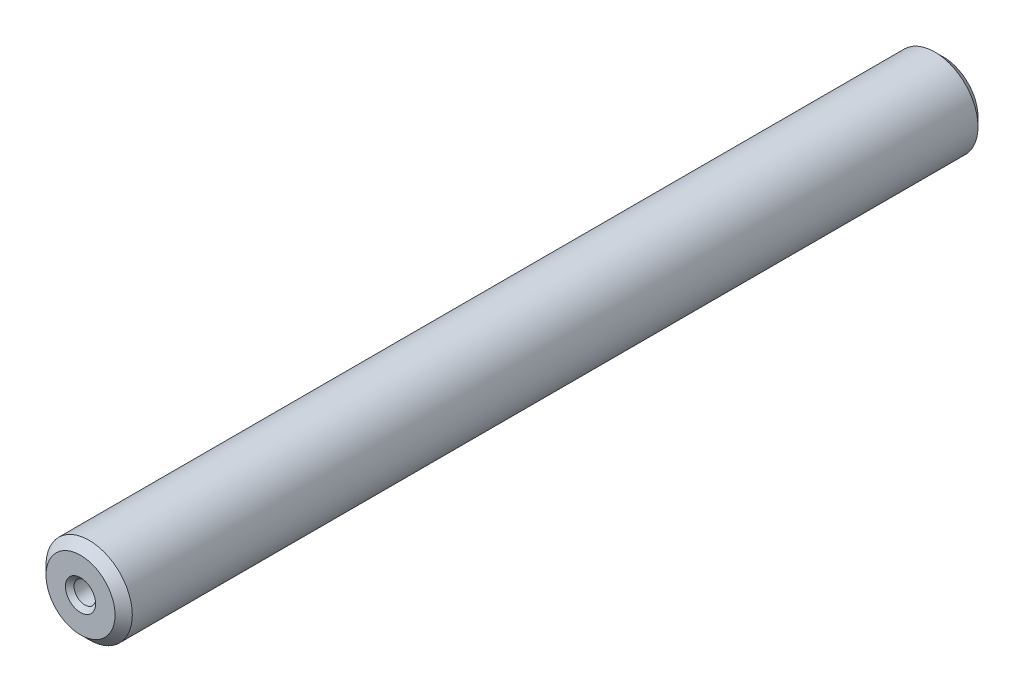
from build123d import *

# Parameters (mm, degrees)
SKETCH1_R             = 5
BOSS_EXTRUDE1_DEPTH   = 100
M3_TAPPED_HOLE1_D     = 2.5
M3_TAPPED_HOLE1_DEPTH = 6.5
M3_TAPPED_HOLE1_TIP   = 0.751075774
CHAMFER1_SIZE         = 1
CHAMFER2_SIZE         = 0.5


with BuildPart() as part:
    # Sketch1 → Boss-Extrude1 (new body)
    with BuildSketch(Plane.XY):
        Circle(SKETCH1_R)
    extrude(amount=BOSS_EXTRUDE1_DEPTH)

    # M3 Tapped Hole1
    with Locations(Plane.XY.offset(100)):
        with Locations((0, 0)):
            Hole(M3_TAPPED_HOLE1_D / 2, depth=M3_TAPPED_HOLE1_DEPTH)
            with Locations((0, 0, -(M3_TAPPED_HOLE1_DEPTH + M3_TAPPED_HOLE1_TIP / 2))):  # 118° drill point
                Cone(0, M3_TAPPED_HOLE1_D / 2, M3_TAPPED_HOLE1_TIP, mode=Mode.SUBTRACT)

    # Chamfer1
    chamfer1_edges = [part.edges().sort_by_distance(p)[0] for p in [
        (-5, 0, 0),
        (-5, 0, 100),
    ]]
    chamfer(chamfer1_edges, length=CHAMFER1_SIZE)

    # Chamfer2
    chamfer2_edges = [part.edges().sort_by_distance(p)[0] for p in [
        (1.25, 0, 100),
    ]]
    chamfer(chamfer2_edges, length=CHAMFER2_SIZE)


solid = part.part
